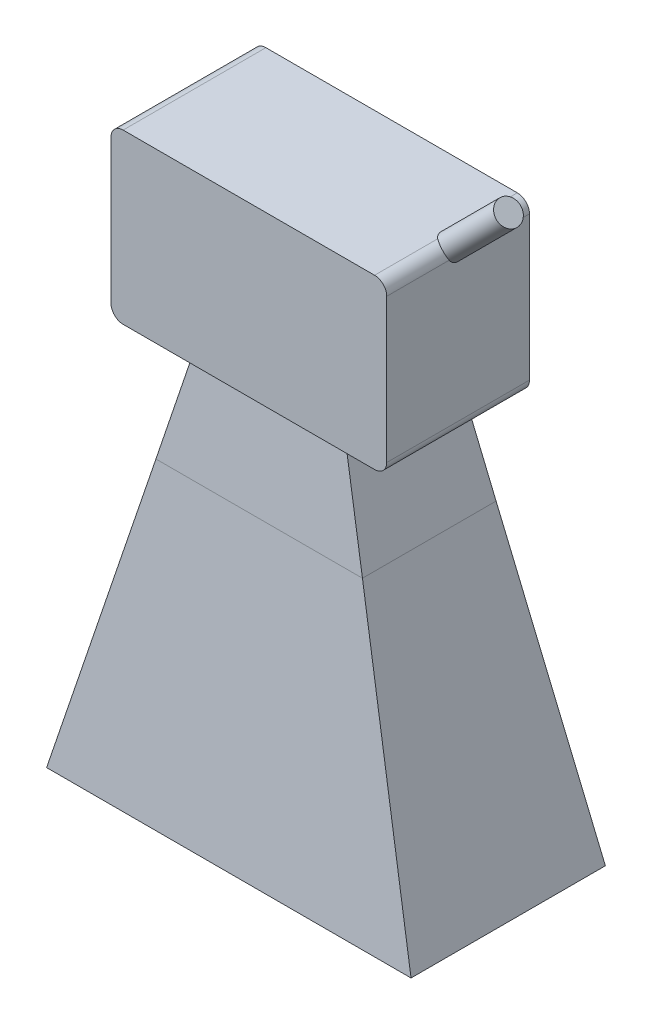
from build123d import *

# Parameters (mm, degrees)
EXTRUDE_1_DEPTH        = 11.75
SKETCH_3_R             = 2
SKETCH_5_R             = 3.75
CUT_EXTRUDE_1_DEPTH    = 5
HOLE_WIZARD_M3_1_D     = 2.5
HOLE_WIZARD_M3_1_DEPTH = 8.5
HOLE_WIZARD_M3_1_TIP   = 0.751075774
SHELL_2_T              = -0.2


with BuildPart() as part:
    # 草图1 → 凸台-拉伸1 (new, symmetric)
    with BuildSketch(Plane.XY):
        with BuildLine():
            Line((-20.7, -13.85), (20.7, -13.85))
            ThreePointArc((20.7, -13.85), (22.114213562, -13.264213562), (22.7, -11.85))
            Line((22.7, -11.85), (22.7, 11.85))
            ThreePointArc((22.7, 11.85), (22.114213562, 13.264213562), (20.7, 13.85))
            Line((20.7, 13.85), (-20.7, 13.85))
            ThreePointArc((-20.7, 13.85), (-22.114213562, 13.264213562), (-22.7, 11.85))
            Line((-22.7, 11.85), (-22.7, -11.85))
            ThreePointArc((-22.7, -11.85), (-22.114213562, -13.264213562), (-20.7, -13.85))
        make_face()
    extrude(amount=EXTRUDE_1_DEPTH, both=True)

    # 扫描1: sweep along a path in 草图2
    with BuildLine(Plane.XY) as sweep_1_path:
        Line((20.32238738, 11.5150831), (30.928989098, 22.121684818))
    # 草图3 → 扫描1 (sweep)
    with BuildSketch(Plane(origin=(30.928989098, 22.121684818, 0), x_dir=(0, 0, -1), z_dir=(0.7071067811865479, 0.7071067811865471, 0))):
        with Locations((0, -0.089229589)):
            Circle(SKETCH_3_R)
    sweep(path=sweep_1_path.line)

    # 草图5 → 切除-拉伸1 (cut)
    with BuildSketch(Plane.XZ.offset(13.85)):
        with Locations(Location((-1.8, -2.75, 0), (0, 0, 270))):
            Circle(SKETCH_5_R)
    extrude(amount=-CUT_EXTRUDE_1_DEPTH, mode=Mode.SUBTRACT)

    # M3 螺纹孔1
    with Locations(Plane(origin=(0, 0, -11.75), x_dir=(-1, 0, 0), z_dir=(0, 0, -1))):
        with Locations((-15.875, 9.35), (15.875, 9.35)):
            Hole(HOLE_WIZARD_M3_1_D / 2, depth=HOLE_WIZARD_M3_1_DEPTH)
            with Locations((0, 0, -(HOLE_WIZARD_M3_1_DEPTH + HOLE_WIZARD_M3_1_TIP / 2))):  # 118° drill point
                Cone(0, HOLE_WIZARD_M3_1_D / 2, HOLE_WIZARD_M3_1_TIP, mode=Mode.SUBTRACT)


with BuildPart() as body_2:
    # 草图9 → 放样5 section 0
    with BuildSketch(Plane(origin=(0, -33.85, 0), x_dir=(-1, 0, 0), z_dir=(0, -1, 0))):
        with BuildLine():
            Line((-15.2, -8.25), (18.8, -8.25))
            Line((18.8, -8.25), (18.8, 13.75))
            Line((18.8, 13.75), (-15.2, 13.75))
            Line((-15.2, 13.75), (-15.2, -8.25))
        make_face()
    # 草图10 → 放样5 section 1
    with BuildSketch(Plane(origin=(0, -81.85, 0), x_dir=(-1, 0, 0), z_dir=(0, -1, 0))):
        with BuildLine():
            Line((-28.2, -13.25), (31.8, -13.25))
            Line((31.8, -13.25), (31.8, 18.75))
            Line((31.8, 18.75), (-28.2, 18.75))
            Line((-28.2, 18.75), (-28.2, -13.25))
        make_face()
    loft()

    # 抽壳2
    shell_2_openings = [body_2.faces().sort_by_distance(p)[0] for p in [
        (-1.8, -81.85, -2.75),
        (-1.8, -33.85, -2.75),
    ]]
    offset(amount=SHELL_2_T, openings=shell_2_openings, kind=Kind.INTERSECTION)


with BuildPart() as body_3:
    # 草图9<5> → 放样6 section 0
    with BuildSketch(Plane(origin=(0, -33.85, 0), x_dir=(-1, 0, 0), z_dir=(0, -1, 0))):
        with BuildLine():
            Line((-15.2, -8.25), (18.8, -8.25))
            Line((18.8, -8.25), (18.8, 13.75))
            Line((18.8, 13.75), (-15.2, 13.75))
            Line((-15.2, 13.75), (-15.2, -8.25))
        make_face()
    # 草图15 → 放样6 section 1
    with BuildSketch(Plane(origin=(0, -13.85, 0), x_dir=(1, 0, 0), z_dir=(0, 1, 0))):
        with BuildLine():
            Line((-13.385, -6.21), (9.785, -6.21))
            Line((9.785, -6.21), (9.785, 11.71))
            Line((9.785, 11.71), (-13.385, 11.71))
            Line((-13.385, 11.71), (-13.385, -6.21))
        make_face()
    loft()


solid = Compound([part.part, body_2.part, body_3.part])
